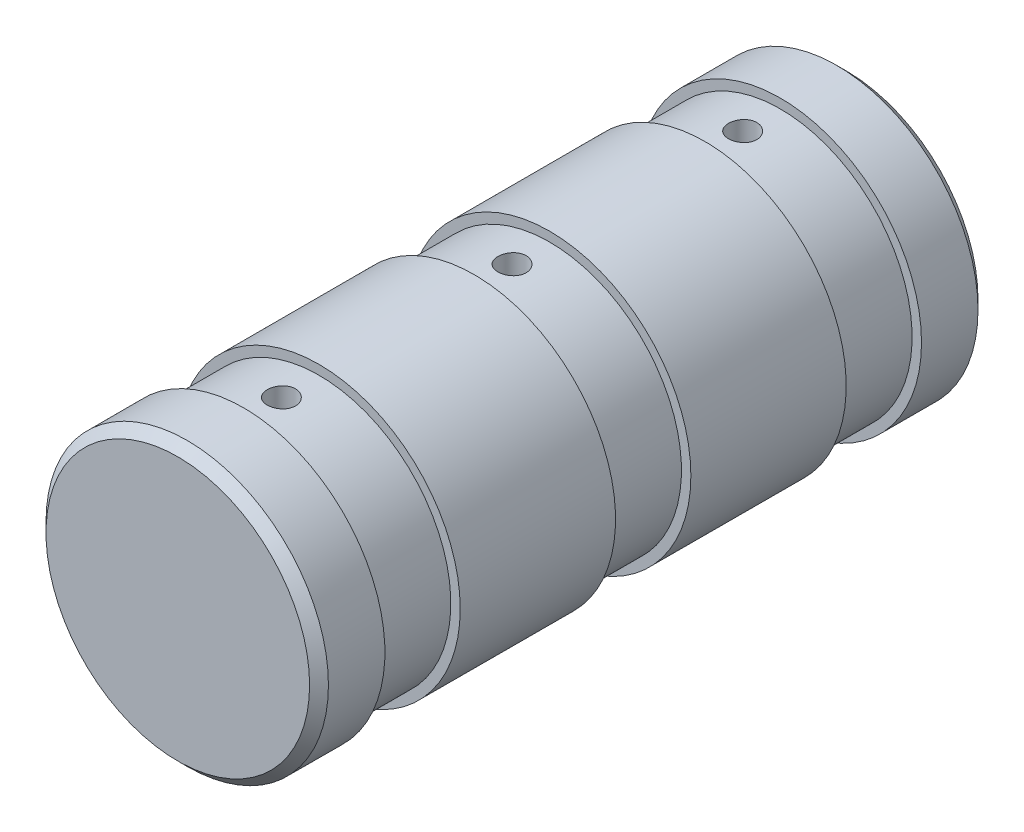
SolidWorks part; units mm, degrees
material "1023 碳钢板 (SS)"
ref_plane "Front Plane" through (0, 0, 0) normal (0, 0, 1) x (1, 0, 0)
ref_plane "Top Plane" through (0, 0, 0) normal (0, 1, 0) x (1, 0, 0)
ref_plane "Right Plane" through (0, 0, 0) normal (1, 0, 0) x (0, 0, -1)
sketch "Sketch1" plane through (0, 0, 0) normal (0, 0, 1) x (1, 0, 0)
  circle A0 centre (0, 0) radius 15
extrude "Boss-Extrude1" add sketch "Sketch1" along normal blind 71
chamfer "Chamfer1" distance 1 angle 45 2 edges at (15, 0, 0) (15, 0, 71)
ref_plane "Plane1" through (0, 15, 0) normal (0, 1, 0) x (1, 0, 0)
sketch "Sketch6" plane through (0, 15, 0) normal (0, 1, 0) x (1, 0, 0)
  line L0 (14, 0) -> (-14, 0) construction
  line L2 (-15, -1) -> (-15, -70) construction
  line L3 (-14, -71) -> (14, -71) construction
  circle A0 centre (0, -11) radius 1.5
  circle A1 centre (0, -35.5) radius 1.5
  circle A2 centre (0, -60) radius 1.5
  dimension "D1" = 11
  dimension "D2" = 15
  dimension "D3" = 35.5
  dimension "D4" = 11
extrude "Cut-Extrude1" cut sketch "Sketch6" against normal blind 17
hole_wizard "Size mm dowel hole 6" positions "Sketch11" profile "Sketch12" hole size "Ø3.0" standard "IS"
sketch "Sketch11" plane through (0, 15, 0) normal (0, 1, 0) x (1, 0, 0)
  point P3 (0, -11)
  point P6 (0, -35.5)
  point P9 (0, -60)
sketch "Sketch12" plane through (0, 15, 11) normal (1, 0, 0) x (0, 0, 1)
  line L0 (0, 0) -> (0, 17.9013)
  line L1 (0, 17.9013) -> (1.5, 17)
  line L2 (1.5, 17) -> (1.5, 0)
  line L5 (1.5, 0) -> (0, 0)
  line L10 (0, 17.9013) -> (-1.5, 17) construction
  line L11 (0, -6.35) -> (0, 107.95) construction
  dimension "孔直径" = 3
  dimension "孔深度" = 17
  dimension "导头角度" = 118
sketch "Sketch17" plane through (0, 0, 0) normal (0, 1, 0) x (1, 0, 0)
  line L0 (15, -70) -> (15, -1) construction
  line L1 (14, -7) -> (16, -7)
  line L2 (14, -7) -> (14, -15)
  line L3 (14, -15) -> (16, -15)
  line L4 (16, -7) -> (16, -15)
  line L5 (14, -7) -> (16, -15) construction
  line L6 (14, -15) -> (16, -7) construction
  line L7 (0, 0) -> (0, -71) construction
  line L8 (-14, -71) -> (14, -71) construction
  line L9 (14, 0) -> (-14, 0) construction
  line L11 (14, -31.5) -> (16, -31.5)
  line L12 (14, -31.5) -> (14, -39.5)
  line L13 (14, -39.5) -> (16, -39.5)
  line L14 (16, -31.5) -> (16, -39.5)
  line L15 (14, -31.5) -> (16, -39.5) construction
  line L16 (14, -39.5) -> (16, -31.5) construction
  line L17 (14, -56) -> (16, -56)
  line L18 (14, -56) -> (14, -64)
  line L19 (14, -64) -> (16, -64)
  line L20 (16, -56) -> (16, -64)
  line L21 (14, -56) -> (16, -64) construction
  line L22 (14, -64) -> (16, -56) construction
  point P0 (15, -11)
  point P12 (15, -35.5)
  point P19 (15, -60)
  dimension "D1" = 8
  dimension "D2" = 2
  dimension "D3" = 11
  dimension "D4" = 2
  dimension "D5" = 8
  dimension "D6" = 8
  dimension "D7" = 2
revolve "Cut-Revolve1" cut sketch "Sketch17" angle 360 about L7
sketch "Sketch19" plane through (0, 0, 0) normal (0, 0, -1) x (-1, 0, 0)
  circle A0 centre (0, 0) radius 1.5
hole_wizard "Size mm dowel hole 7" positions "3DSketch15" profile "Sketch24" hole size "Ø3.0" standard "IS"
sketch3d "3DSketch15"
  point P0 (0, 0, 0)
sketch "Sketch24" plane through (0, 0, 0) normal (1, 0, 0) x (0, 1, 0)
  line L0 (0, 0) -> (0, 62.9013)
  line L1 (0, 62.9013) -> (1.5, 62)
  line L2 (1.5, 62) -> (1.5, 0)
  line L5 (1.5, 0) -> (0, 0)
  line L10 (0, 62.9013) -> (-1.5, 62) construction
  line L11 (0, -6.35) -> (0, 107.95) construction
  dimension "孔直径" = 3
  dimension "孔深度" = 62
  dimension "导头角度" = 118
hole_wizard "M4 Tapped Hole1" positions "3DSketch22" profile "Sketch29" tap size "M4" standard "IS"
sketch3d "3DSketch22"
  point P0 (0, 0, 0)
sketch "Sketch29" plane through (0, 0, 0) normal (1, 0, 0) x (0, 1, 0)
  line L0 (0, 0) -> (0, 6)
  line L1 (0, 6) -> (1.65, 5.0086)
  line L2 (1.65, 5.0086) -> (1.65, 0)
  line L5 (1.65, 0) -> (0, 0)
  line L10 (0, 6) -> (-1.65, 5.0086) construction
  line L11 (0, -6.35) -> (0, 107.95) construction
  dimension "螺纹孔钻头直径" = 3.3
  dimension "螺纹孔钻头深度" = 6
  dimension "导头角度" = 118
cosmetic thread "Hole thread 1" parameters "D1"=8, "D2"=4
